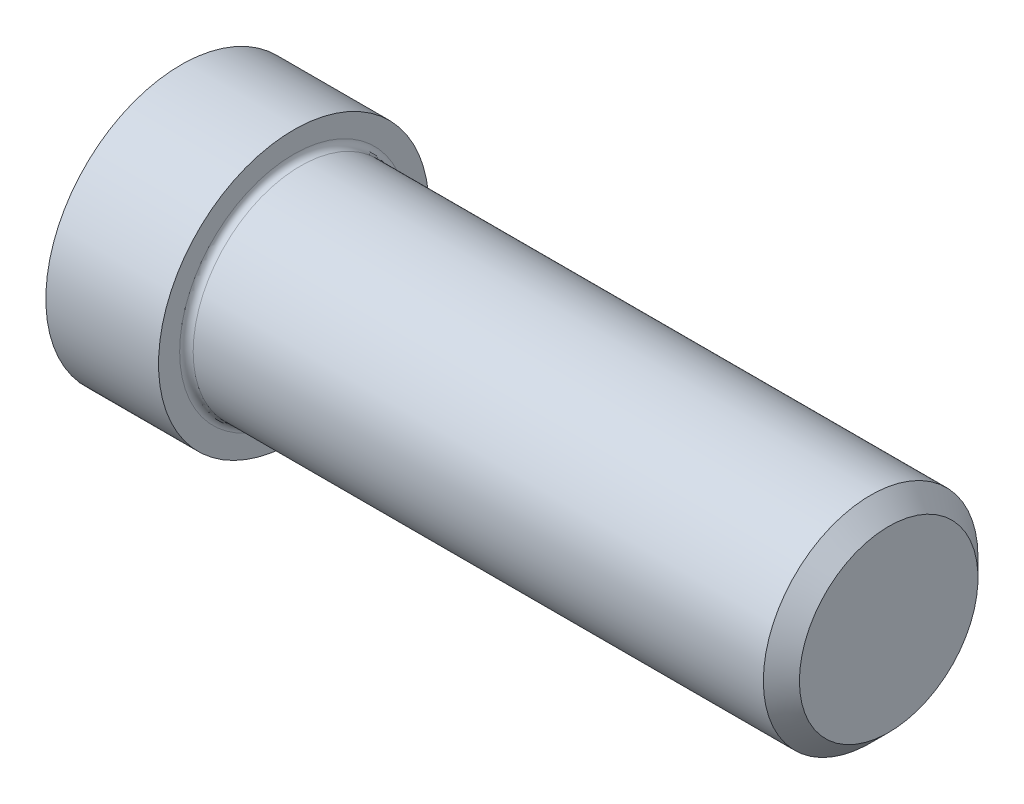
SolidWorks part; units mm, degrees
material "SAE5"
ref_plane "Front" through (0, 0, 0) normal (0, 0, 1) x (1, 0, 0)
ref_plane "Top" through (0, 0, 0) normal (0, 1, 0) x (1, 0, 0)
ref_plane "Right" through (0, 0, 0) normal (1, 0, 0) x (0, 0, -1)
sketch "Sketch1" plane through (0, 0, 0) normal (1, 0, 0) x (0, 0, -1)
  line L0 (12, 6.9282) -> (12, -6.9282) construction
  line L1 (-12, 6.9282) -> (-12, -6.9282) construction
  line L2 (12, -6.9282) -> (0, -13.8564) construction
  line L3 (0, -13.8564) -> (-12, -6.9282) construction
  line L4 (12, 6.9282) -> (0, 13.8564) construction
  line L5 (0, 13.8564) -> (-12, 6.9282) construction
  line L6 (-14.9874, 0) -> (25.9385, 0) construction
  line L7 (0, 19.0954) -> (0, -18.9245) construction
  circle A0 centre (0, 0) radius 12
  dimension "D1" = 13.8564
  dimension "s" = 24
  dimension "D2" = 120
extrude "Base-Extrude" add sketch "Sketch1" along normal blind 10
sketch "Sketch2" plane through (0, 0, 0) normal (0, 0, 1) x (1, 0, 0)
  line L0 (10, -12) -> (10, 12) construction
  line L1 (0, 0) -> (62.8, 0)
  line L2 (0, 0) -> (0, 9.525)
  line L3 (0, 9.525) -> (27.8072, 9.525)
  line L4 (62.8, 0) -> (62.8, 6.268)
  line L7 (0, 0) -> (96.52, 0) construction
  line L8 (62.8, -6.268) -> (27.8072, -9.525) construction
  line L9 (0, -9.525) -> (27.8072, -9.525) construction
  line L10 (12, 15.24) -> (12, -1.27) construction
  line L11 (17.8, 15.24) -> (17.8, -1.27) construction
  line L13 (27.8072, 9.525) -> (62.8, 9.525)
  line L14 (62.8, 9.525) -> (62.8, 6.268)
  dimension "D1" = 2
  dimension "m" = 19.05
  dimension "Minor_dia" = 12.536
  dimension "h" = 45
  dimension "D2" = 50.8
revolve "Boss-Revolve1" add sketch "Sketch2" angle 360 about L7
cosmetic thread "Helix1" parameters "Thread_length"=25.4, "Thread_minor"=12.536
chamfer "Chamfer" distance 1.6 angle 45 1 edges at (62.8, 0, 9.525)
fillet "Fillet" radius 0.6 1 edges at (10, 0, -9.525)
sketch "Sketch6" plane through (0, 0, 0) normal (0, 0, 1) x (1, 0, 0)
  line L0 (65, -6.268) -> (64, -8)
  line L1 (65, -6.268) -> (66, -8)
  line L2 (66, -8) -> (66, -10)
  line L3 (-3.175, 0) -> (5.1513, 0) construction
  line L5 (66, -10) -> (64, -10)
  line L6 (64, -10) -> (64, -8)
  dimension "Thread_minor" = 12.536
  dimension "Diameter" = 16
  dimension "Start" = 65
  dimension "SideAngle" = 60
  dimension "VeeAngle" = 60
  dimension "Overcut" = 20
revolve "Cut-Revolve4" [suppressed] cut sketch "Sketch6" angle 360 about L3
pattern_linear "LPattern1" [suppressed]
sketch "Sketch7" plane through (0, 0, 0) normal (-1, 0, 0) x (0, 0, 1)
  line L0 (0, 12.4766) -> (0, -13.45) construction
  line L1 (-12.9191, 0) -> (14.8215, 0) construction
  line L2 (-8.7679, 5.0621) -> (-8.7679, -5.0621)
  line L3 (-8.7679, -5.0621) -> (0, -10.1243)
  line L4 (0, -10.1243) -> (8.7679, -5.0621)
  line L5 (8.7679, -5.0621) -> (8.7679, 5.0621)
  line L6 (8.7679, 5.0621) -> (0, 10.1243)
  line L7 (0, 10.1243) -> (-8.7679, 5.0621)
  dimension "D1" = 10.1243
  dimension "D2" = 120
extrude "Cut-Extrude1" cut sketch "Sketch7" against normal blind 7.62
